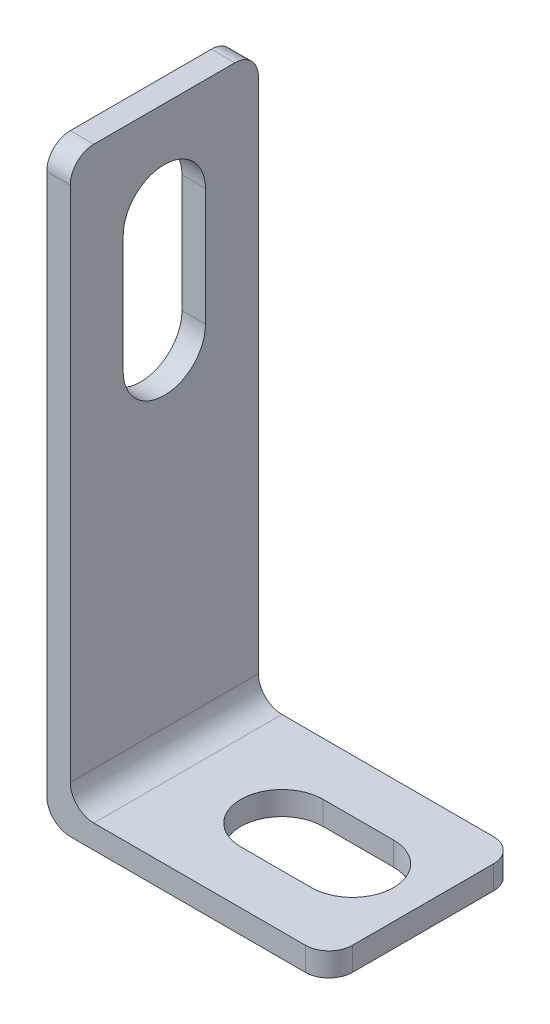
from build123d import *

# Parameters (mm, degrees)
EXTRUDE_THIN1_DEPTH = 4
CUT_EXTRUDE1_DEPTH  = 28.129319933
CUT_EXTRUDE2_DEPTH  = 29.017851452
FILLET1_R           = 1


with BuildPart() as part:
    # Sketch1 → Extrude-Thin1 (new, symmetric)
    with BuildSketch(Plane.XY):
        Polygon((12, 0), (0, 0), (0, 25), (1, 25), (1, 1), (12, 1), align=None)
    extrude(amount=EXTRUDE_THIN1_DEPTH, both=True)

    # Sketch2 → Cut-Extrude1 (cut, through all)
    with BuildSketch(Plane(origin=(0, 1, 0), x_dir=(1, 0, 0), z_dir=(0, 1, 0))):
        with BuildLine():
            Line((6, 1.75), (9, 1.75))
            ThreePointArc((9, 1.75), (10.75, 0), (9, -1.75))
            Line((9, -1.75), (6, -1.75))
            ThreePointArc((6, -1.75), (4.25, 0), (6, 1.75))
        make_face()
    extrude(amount=-CUT_EXTRUDE1_DEPTH, mode=Mode.SUBTRACT)

    # Sketch3 → Cut-Extrude2 (cut, through all)
    with BuildSketch(Plane.ZY):
        with BuildLine():
            Line((-1.75, 16), (-1.75, 21))
            ThreePointArc((-1.75, 21), (0, 22.75), (1.75, 21))
            Line((1.75, 21), (1.75, 16))
            ThreePointArc((1.75, 16), (0, 14.25), (-1.75, 16))
        make_face()
    extrude(amount=-CUT_EXTRUDE2_DEPTH, mode=Mode.SUBTRACT)

    # Fillet1
    fillet1_edges = [part.edges().sort_by_distance(p)[0] for p in [
        (0.5, 25, 4),
        (0.5, 25, -4),
        (12, 0.5, -4),
        (12, 0.5, 4),
        (0, 0, 0),
        (1, 1, 0),
    ]]
    fillet(fillet1_edges, radius=FILLET1_R)


solid = part.part
